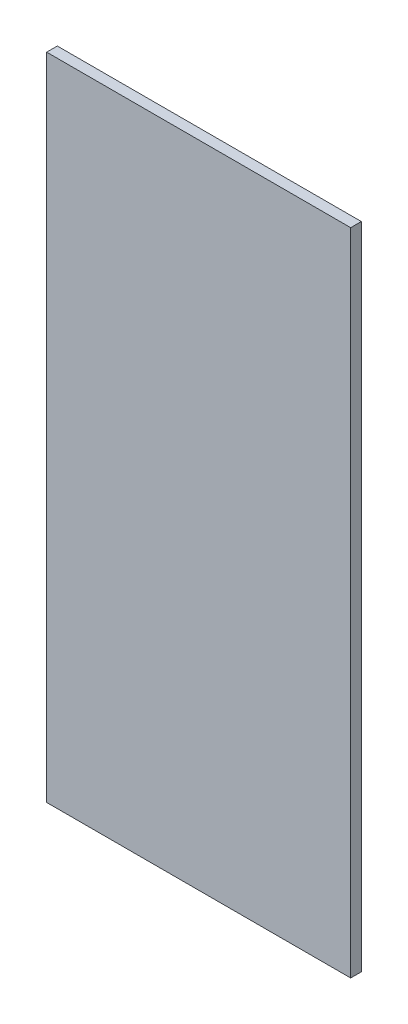
SolidWorks part; units mm, degrees
material "普通碳钢"
ref_plane "Front Plane" through (0, 0, 0) normal (0, 0, 1) x (1, 0, 0)
ref_plane "Top Plane" through (0, 0, 0) normal (0, 1, 0) x (1, 0, 0)
ref_plane "Right Plane" through (0, 0, 0) normal (1, 0, 0) x (0, 0, -1)
sketch "Sketch1" plane through (0, 0, 0) normal (0, 0, 1) x (1, 0, 0)
  line L1 (-200, 427.5) -> (200, 427.5)
  line L2 (-200, 427.5) -> (-200, -427.5)
  line L3 (-200, -427.5) -> (200, -427.5)
  line L4 (200, 427.5) -> (200, -427.5)
  dimension "D1" = 855
  dimension "D2" = 400
  dimension "D3" = 427.5
  dimension "D4" = 200
extrude "Boss-Extrude1" add sketch "Sketch1" along normal mid plane 14
